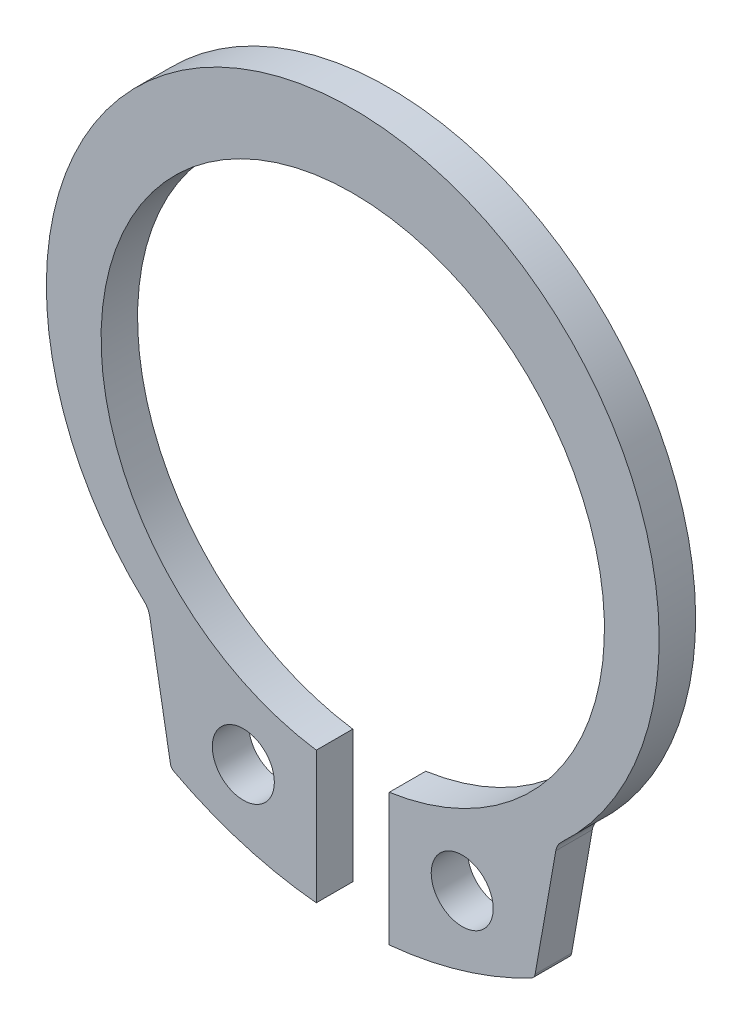
from build123d import *

# Parameters (mm, degrees)
EXTRUDE_972_DEPTH      = 0.5
EXTRUDE_972_DEPTH_BACK = 0.5
SKETCH_1_R             = 0.85


with BuildPart() as part:
    # 草图1 → Extrude 972 (new, two sides: drawn at the far end of the back side and taken through both)
    with BuildSketch(Plane.XY.offset(-EXTRUDE_972_DEPTH_BACK)):
        with BuildLine():
            Line((-1, -7.327151675), (-1, -10.95227248))
            ThreePointArc((-1, -10.95227248), (-3.005026441, -10.560805936), (-4.896301332, -9.788500055))
            ThreePointArc((-4.896301332, -9.788500055), (-4.964631615, -9.729422113), (-5, -9.64630588))
            Line((-5, -9.64630588), (-5.566746879, -6.432124609))
            ThreePointArc((-5.566746879, -6.432124609), (-5.619937096, -6.280010711), (-5.718749028, -6.152715625))
            ThreePointArc((-5.718749028, -6.152715625), (0, 8.4), (5.718749028, -6.152715625))
            ThreePointArc((5.718749028, -6.152715625), (5.619937096, -6.280010711), (5.566746879, -6.432124609))
            Line((5.566746879, -6.432124609), (5, -9.64630588))
            ThreePointArc((5, -9.64630588), (4.964631615, -9.729422113), (4.896301332, -9.788500055))
            ThreePointArc((4.896301332, -9.788500055), (3.005026441, -10.560805936), (1, -10.95227248))
            Line((1, -10.95227248), (1, -7.327151675))
            ThreePointArc((1, -7.327151675), (0, 6.4), (-1, -7.327151675))
        make_face()
        with Locations((-3, -8.666394553)):
            Circle(SKETCH_1_R, mode=Mode.SUBTRACT)
        with Locations(Location((3, -8.666394553, 0), (0, 0, 180))):
            Circle(SKETCH_1_R, mode=Mode.SUBTRACT)
    extrude(amount=EXTRUDE_972_DEPTH + EXTRUDE_972_DEPTH_BACK)


solid = part.part
